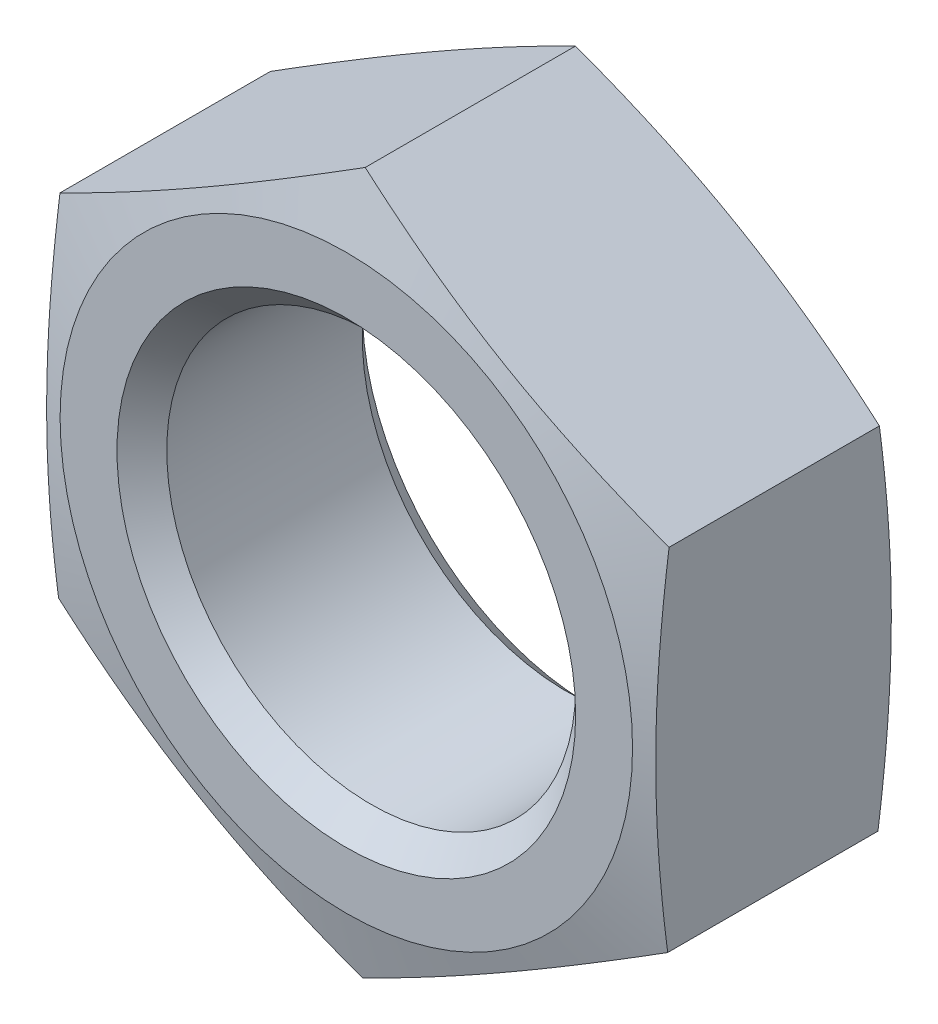
from build123d import *

# Parameters (mm, degrees)
SKETCH1_R          = 12.5
BASE_EXTRUDE_DEPTH = 15
SKETCH2_OUTSIDE_W  = 298.754
SKETCH2_OUTSIDE_H  = 304.43
SKETCH2_OUTSIDE_R  = 17.5
CUT_EXTRUDE1_DEPTH = 33.179208695
CUT_EXTRUDE1_DRAFT = -75
SKETCH3_OUTSIDE_W  = 298.754
SKETCH3_OUTSIDE_H  = 304.43
SKETCH3_OUTSIDE_R  = 17.5
CUT_EXTRUDE2_DEPTH = 33.179208695
CUT_EXTRUDE2_DRAFT = -75
CHAMFER1_SIZE      = 1.521428571


with BuildPart() as part:
    # Sketch1 → Base-Extrude (new body)
    with BuildSketch(Plane.XY):
        Polygon((0.084573131, 21.499833659), (-18.577115561, 10.823159309), (-18.661688692, -10.67667435), (-0.084573131, -21.499833659), (18.577115561, -10.823159309), (18.661688692, 10.67667435), align=None)
        Circle(SKETCH1_R, mode=Mode.SUBTRACT)
    extrude(amount=BASE_EXTRUDE_DEPTH)


with BuildPart() as cut_extrude1_tool:
    # Sketch2 outside → Cut-Extrude1 (with draft: the straight prism first)
    with BuildSketch(Plane(origin=(0, 0, 0), x_dir=(-1, 0, 0), z_dir=(0, 0, -1))):
        Rectangle(SKETCH2_OUTSIDE_W, SKETCH2_OUTSIDE_H)
        Circle(SKETCH2_OUTSIDE_R, mode=Mode.SUBTRACT)
    extrude(amount=-CUT_EXTRUDE1_DEPTH)
    # Cut-Extrude1: the draft: its side faces are tilted about the plane it starts from
    cut_extrude1_sides = [cut_extrude1_tool.faces().sort_by_distance(p)[0] for p in [
        (0, -152.215, 16.589604347),
        (-149.377, 0, 16.589604347),
        (0, 152.215, 16.589604347),
        (149.377, 0, 16.589604347),
        (17.5, 0, 16.589604347),
    ]]
    draft(cut_extrude1_sides, Plane(origin=(0, 0, 0), x_dir=(-1, 0, 0), z_dir=(0, 0, -1)), CUT_EXTRUDE1_DRAFT)


with BuildPart() as part_1:
    add(part.part)

    # Cut-Extrude1: cut by cut_extrude1_tool
    add(cut_extrude1_tool.part, mode=Mode.SUBTRACT)


with BuildPart() as cut_extrude2_tool:
    # Sketch3 outside → Cut-Extrude2 (with draft: the straight prism first)
    with BuildSketch(Plane.XY.offset(15)):
        Rectangle(SKETCH3_OUTSIDE_W, SKETCH3_OUTSIDE_H)
        Circle(SKETCH3_OUTSIDE_R, mode=Mode.SUBTRACT)
    extrude(amount=-CUT_EXTRUDE2_DEPTH)
    # Cut-Extrude2: the draft: its side faces are tilted about the plane it starts from
    cut_extrude2_sides = [cut_extrude2_tool.faces().sort_by_distance(p)[0] for p in [
        (0, -152.215, -1.589604347),
        (149.377, 0, -1.589604347),
        (0, 152.215, -1.589604347),
        (-149.377, 0, -1.589604347),
        (-17.5, 0, -1.589604347),
    ]]
    draft(cut_extrude2_sides, Plane.XY.offset(15), CUT_EXTRUDE2_DRAFT)


with BuildPart() as part_2:
    add(part_1.part)

    # Cut-Extrude2: cut by cut_extrude2_tool
    add(cut_extrude2_tool.part, mode=Mode.SUBTRACT)

    # Chamfer1
    chamfer1_edges = [part_2.edges().sort_by_distance(p)[0] for p in [
        (-12.5, 0, 0),
        (-12.5, 0, 15),
    ]]
    chamfer(chamfer1_edges, length=CHAMFER1_SIZE)


solid = part_2.part
